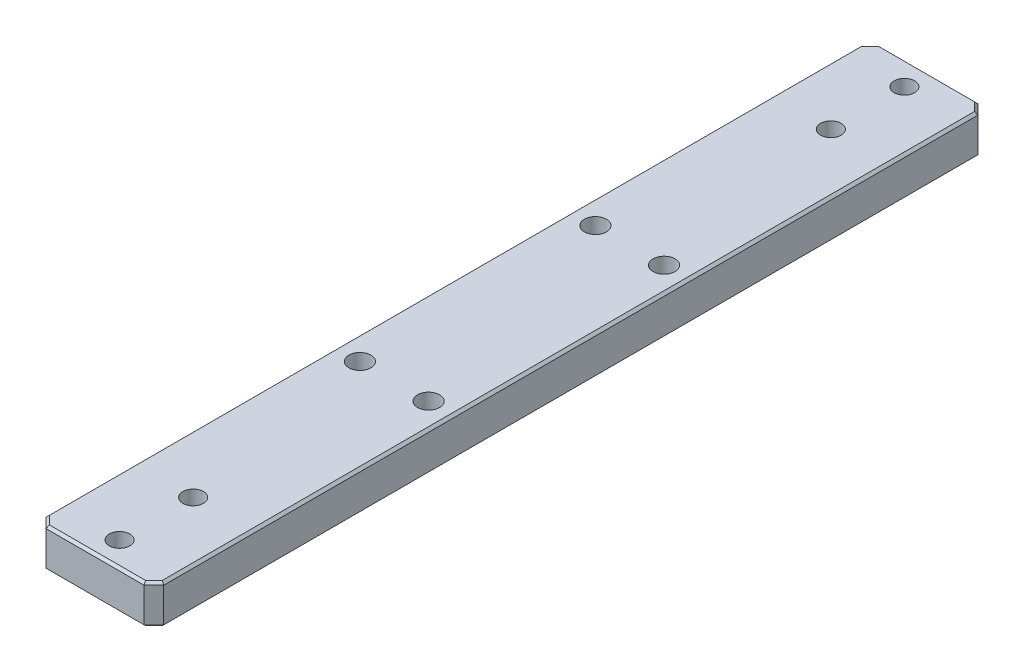
from build123d import *

# Parameters (mm, degrees)
SKETCH_1_W                   = 24
SKETCH_1_H                   = 170
EXTRUDE_1_DEPTH              = 8
HOLE_WIZARD_M4_1_D           = 4.5
HOLE_WIZARD_M4_1_CBORE_D     = 8
HOLE_WIZARD_M4_1_CBORE_DEPTH = 4.4
HOLE_WIZARD_M5_1_D           = 4.2
HOLE_WIZARD_M5_1_DEPTH       = 12.4
HOLE_WIZARD_M5_1_TIP         = 1.2618073
CHAMFER_1_SIZE               = 2
CHAMFER_2_SIZE               = 0.5


with BuildPart() as part:
    # 草图1 → 凸台-拉伸1 (new body)
    with BuildSketch(Plane(origin=(0, 0, 0), x_dir=(1, 0, 0), z_dir=(0, 1, 0))):
        Rectangle(SKETCH_1_W, SKETCH_1_H)
    extrude(amount=EXTRUDE_1_DEPTH)

    # M4 六角凹头螺钉的柱形沉头孔1 (through all)
    with Locations(Plane(origin=(0, 0, 0), x_dir=(-1, 0, 0), z_dir=(0, -1, 0))):
        with Locations((-7, 24), (7, 24), (-7, -24), (7, -24)):
            CounterBoreHole(HOLE_WIZARD_M4_1_D / 2, HOLE_WIZARD_M4_1_CBORE_D / 2, HOLE_WIZARD_M4_1_CBORE_DEPTH)

    # M5 螺纹孔1
    with Locations(Plane(origin=(0, 8, 0), x_dir=(1, 0, 0), z_dir=(0, 1, 0))):
        with Locations((0, 80), (0, -80), (0, -65), (0, 65)):
            Hole(HOLE_WIZARD_M5_1_D / 2, depth=HOLE_WIZARD_M5_1_DEPTH)
            with Locations((0, 0, -(HOLE_WIZARD_M5_1_DEPTH + HOLE_WIZARD_M5_1_TIP / 2))):  # 118° drill point
                Cone(0, HOLE_WIZARD_M5_1_D / 2, HOLE_WIZARD_M5_1_TIP, mode=Mode.SUBTRACT)

    # 倒角1
    chamfer_1_edges = [part.edges().sort_by_distance(p)[0] for p in [
        (12, 4, 85),
        (-12, 4, 85),
        (-12, 4, -85),
        (12, 4, -85),
    ]]
    chamfer(chamfer_1_edges, length=CHAMFER_1_SIZE)

    # 倒角2
    chamfer_2_edges = [part.edges().sort_by_distance(p)[0] for p in [
        (-12, 0, 0),
        (-12, 8, 0),
        (12, 0, 0),
        (0, 0, 85),
        (0, 0, -85),
        (11, 0, 84),
        (-11, 0, 84),
        (11, 0, -84),
        (-11, 0, -84),
        (0, 8, -85),
        (12, 8, 0),
        (0, 8, 85),
        (11, 8, 84),
        (-11, 8, 84),
        (11, 8, -84),
        (-11, 8, -84),
    ]]
    chamfer(chamfer_2_edges, length=CHAMFER_2_SIZE)


solid = part.part
